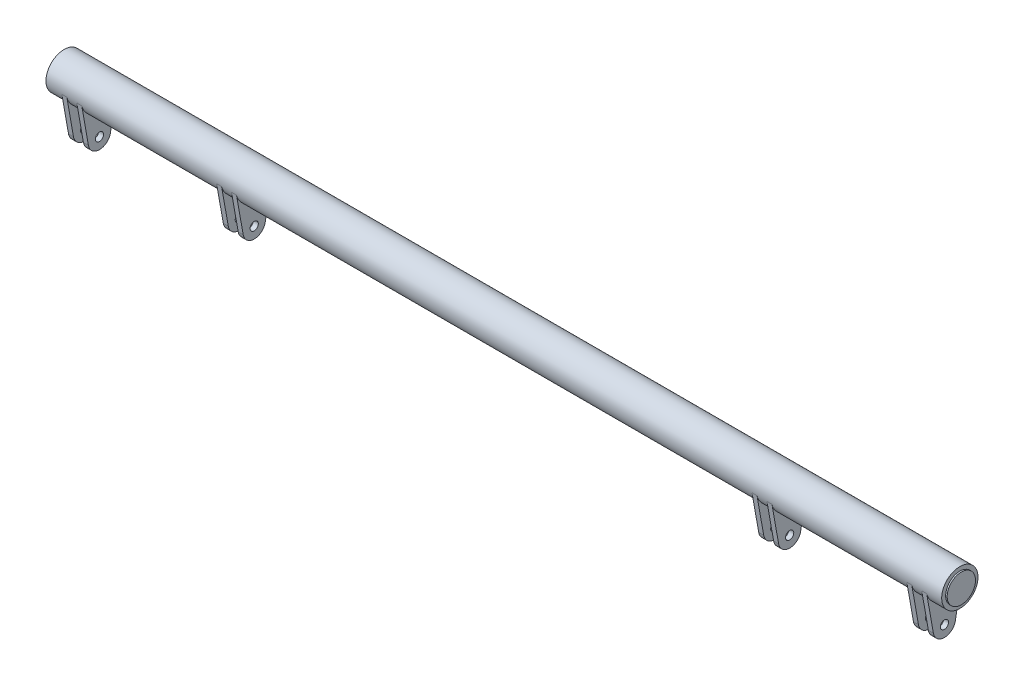
SolidWorks part; units mm, degrees
material "K"
ref_plane "Front" through (0, 0, 0) normal (0, 0, 1) x (1, 0, 0)
ref_plane "Top" through (0, 0, 0) normal (0, 1, 0) x (1, 0, 0)
ref_plane "Right" through (0, 0, 0) normal (1, 0, 0) x (0, 0, -1)
sketch "草图1" plane through (0, 0, 0) normal (0, 0, 1) x (1, 0, 0)
  line L0 (-900, 133.5616) -> (900, 133.5616)
  line L1 (0, 0) -> (0, 532.4658) construction
  dimension "D1" = 1800
other "Structural Member1"
ref_plane "Plane1" through (-900, 133.5616, 0) normal (1, 0, 0) x (0, 1, 0)
sketch "Sketch1" plane through (-900, 133.5616, 0) normal (1, 0, 0) x (0, 1, 0)
  circle A0 centre (0, 0) radius 28.5
  circle A1 centre (0, 0) radius 36.5
  point P3 (-28.5, 0)
  point P5 (-36.5, 0)
  point P6 (28.5, 0)
  point P7 (36.5, 0)
  point P8 (0, 36.5)
  point P9 (0, 28.5)
  point P10 (0, -28.5)
  point P11 (0, -36.5)
  point P12 (0, 0)
  dimension "D" = 73
  dimension "t" = 8
ref_plane "Plane2" through (538, 0, 0) normal (1, 0, 0) x (0, 0, -1)
sketch "Sketch3" plane through (538, 0, 0) normal (1, 0, 0) x (0, 0, -1)
  line L0 (0, 0) -> (0, 532.4658) construction
  line L1 (-35.5842, 125.1908) -> (-22.1528, 49.6241)
  line L2 (0, 53.5616) -> (0, 133.5616) construction
  line L3 (35.0678, 123.239) -> (21.9019, 48.4083)
  arc A0 (-22.1528, 49.6241) -> (21.9019, 48.4083) centre (0, 53.5616) ccw
  circle A1 centre (0, 133.5616) radius 36.5 construction
  circle A2 centre (0, 133.5616) radius 36.5555
  dimension "D1" = 80
  dimension "D2" = 22.5
extrude "Boss-Extrude1" add sketch "Sketch3" along normal blind 10 from offset 10 separate body
hole_wizard "Ø16.5 (16.5) Diameter Hole1" positions "Sketch6" profile "Sketch4" hole size "Ø16.5" standard "GB" end condition up to next
sketch "Sketch6" plane through (558, 0, 0) normal (1, 0, 0) x (0, 0, -1)
  point P0 (0, 53.5616)
sketch "Sketch4" plane through (558, 53.5616, 0) normal (0, 1, 0) x (0, 0, -1)
  line L0 (0, 0) -> (0, 10.001)
  line L1 (0, 10.001) -> (8.25, 10.001)
  line L2 (8.25, 10.001) -> (8.25, 0)
  line L5 (8.25, 0) -> (0, 0)
  line L11 (0, -6.35) -> (0, 107.95) construction
  dimension "通孔孔直径" = 16.5
  dimension "通孔孔深度" = 10.001
pattern_linear "LPattern1" count 2 spacing 30 along (-1, 0, 0) of bodies 103
mirror "Mirror1" about plane through (0, 0, 0) normal (1, 0, 0) of bodies 104 103
pattern_linear "LPattern2" count 2 spacing 311 along (1, 0, 0) of bodies 104 103
mirror "Mirror2" about plane through (0, 0, 0) normal (1, 0, 0) of bodies 108 107
sketch "Sketch7" plane through (-900, 0, 0) normal (-1, 0, 0) x (0, 0, 1)
  circle A0 centre (0, 133.5616) radius 28.5
extrude "Boss-Extrude2" add sketch "Sketch7" along normal blind 3 separate body
sketch "Sketch8" plane through (900, 0, 0) normal (1, 0, 0) x (0, 0, -1)
  circle A0 centre (0, 133.5616) radius 28.5
extrude "Boss-Extrude3" add sketch "Sketch8" along normal blind 3 separate body
equation "\"零件重量\"= IIF ( \"SW-质量\" > 100 , int ( \"SW-质量\" ) , \"SW-质量\" )"
